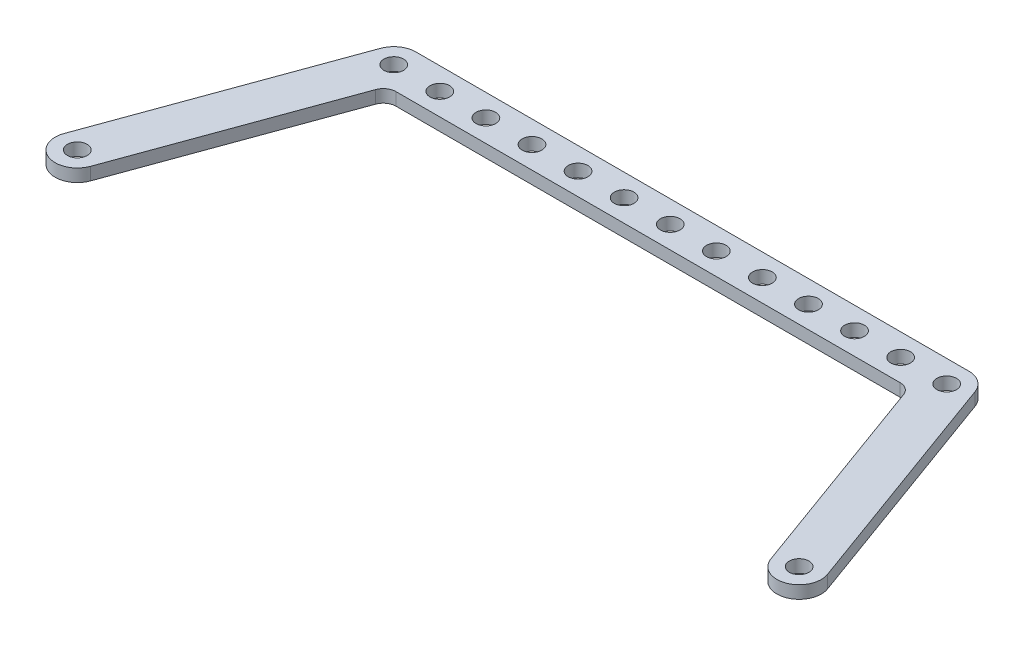
SolidWorks part; units mm, degrees
material "Thornel Mat VMA"
ref_plane "前视基准面" through (0, 0, 0) normal (0, 0, 1) x (1, 0, 0)
ref_plane "上视基准面" through (0, 0, 0) normal (0, 1, 0) x (1, 0, 0)
ref_plane "右视基准面" through (0, 0, 0) normal (1, 0, 0) x (0, 0, -1)
other "Configuration Table"
sketch "草图1" plane through (0, 0, 0) normal (0, 1, 0) x (1, 0, 0)
  line L0 (0, 0) -> (57, 0) construction
  line L1 (0, 0) -> (43.6645, 36.6389) construction
  line L2 (0, 0) -> (0, 57) construction
  line L3 (43.6645, 36.6389) -> (57, 0) construction
  line L4 (46.9535, 37.836) -> (60.2889, 1.1971)
  line L5 (40.3756, 35.4418) -> (53.7111, -1.1971)
  line L6 (-43.6645, 36.6389) -> (43.6645, 36.6389) construction
  line L7 (-43.6645, 40.1389) -> (43.6645, 40.1389)
  line L8 (-43.6645, 33.1389) -> (43.6645, 33.1389)
  line L9 (-57, 0) -> (-43.6645, 36.6389) construction
  line L10 (-60.2889, 1.1971) -> (-46.9535, 37.836)
  line L11 (-53.7111, -1.1971) -> (-40.3756, 35.4418)
  circle A0 centre (0, 0) radius 57 construction
  circle A1 centre (43.6645, 36.6389) radius 1.55
  circle A2 centre (57, 0) radius 1.55
  circle A3 centre (-57, 0) radius 1.55
  circle A4 centre (-43.6645, 36.6389) radius 1.55
  arc A5 (46.9535, 37.836) -> (40.3756, 35.4418) centre (43.6645, 36.6389) ccw
  arc A6 (53.7111, -1.1971) -> (60.2889, 1.1971) centre (57, 0) ccw
  arc A7 (-43.6645, 40.1389) -> (-43.6645, 33.1389) centre (-43.6645, 36.6389) ccw
  arc A8 (43.6645, 33.1389) -> (43.6645, 40.1389) centre (43.6645, 36.6389) ccw
  arc A9 (-60.2889, 1.1971) -> (-53.7111, -1.1971) centre (-57, 0) ccw
  arc A10 (-40.3756, 35.4418) -> (-46.9535, 37.836) centre (-43.6645, 36.6389) ccw
  circle A12 centre (0, 36.6389) radius 1.55
  circle A18 centre (-36.3875, 36.6389) radius 1.55
  circle A19 centre (-29.1105, 36.6389) radius 1.55
  circle A20 centre (-21.8335, 36.6389) radius 1.55
  circle A21 centre (-14.5565, 36.6389) radius 1.55
  circle A22 centre (-7.2795, 36.6389) radius 1.55
  circle A23 centre (7.2795, 36.6389) radius 1.55
  circle A24 centre (14.5565, 36.6389) radius 1.55
  circle A25 centre (21.8335, 36.6389) radius 1.55
  circle A26 centre (29.1105, 36.6389) radius 1.55
  circle A27 centre (36.3875, 36.6389) radius 1.55
  point P12 (50.3323, 18.3194)
  point P17 (0, 36.6389)
  point P23 (-50.3323, 18.3194)
  dimension "D1" = 114
  dimension "D3" = 3.1
  dimension "D4" = 3.5
  dimension "D6" = 7.277
  dimension "D2" = 40
  dimension "D5" = 6
extrude "凸台-拉伸1" add sketch "草图1" along normal blind 2 contours L10 A9 L11 L8 A7 A3 | A10 L11 L8 L5 A5 L7 | L11 A10 A7 L8 A4 | A8 L8 L5 A6 L4 A2 | L8 A8 A5 L5 A1
fillet "圆角1" radius 2 2 edges at (41.2138, 1, -33.1389) (-41.2138, 1, -33.1389)
